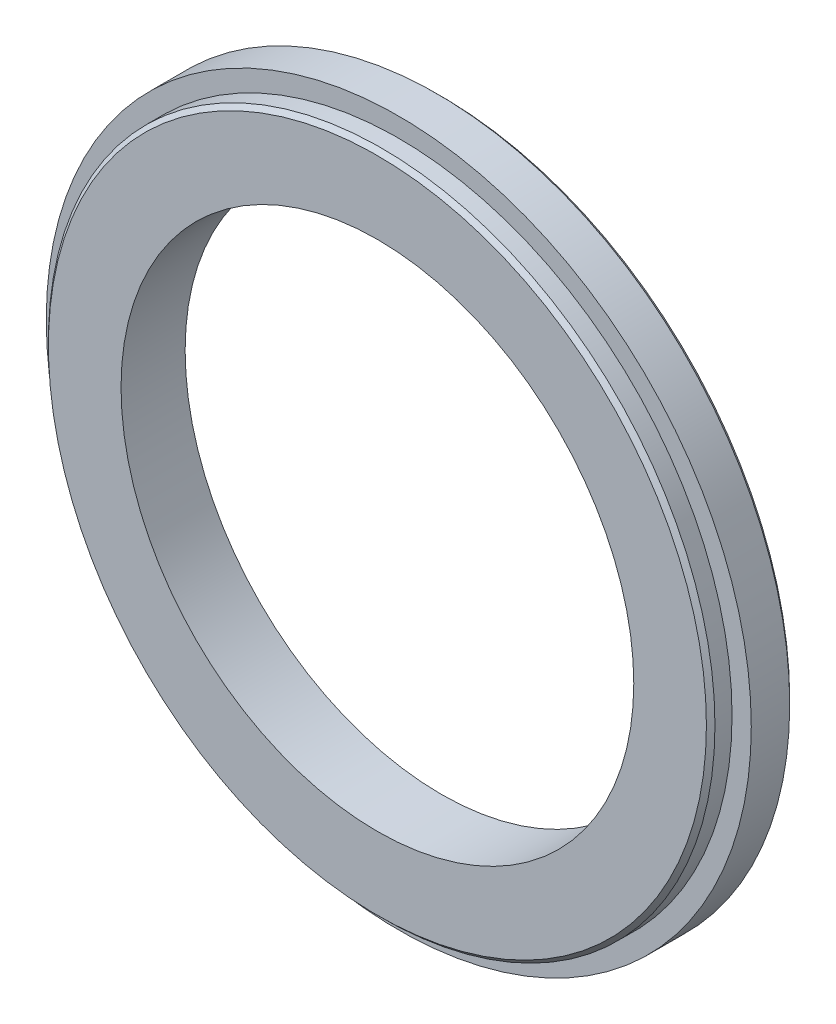
SolidWorks part; units mm, degrees
material "Plain carbon steel"
ref_plane "Front Plane" through (0, 0, 0) normal (0, 0, 1) x (1, 0, 0)
ref_plane "Top Plane" through (0, 0, 0) normal (0, 1, 0) x (1, 0, 0)
ref_plane "Right Plane" through (0, 0, 0) normal (1, 0, 0) x (0, 0, -1)
sketch "Sketch1" plane through (0, 0, 0) normal (0, 0, 1) x (1, 0, 0)
  circle A0 centre (0, 0) radius 82.5
  circle A1 centre (0, 0) radius 60
extrude "Boss-Extrude1" add sketch "Sketch1" along normal blind 10
sketch "Sketch2" plane through (0, 0, 10) normal (0, 0, 1) x (1, 0, 0)
  circle A0 centre (0, 0) radius 78
  circle A1 centre (0, 0) radius 60
extrude "Boss-Extrude2" add sketch "Sketch2" along normal blind 5
chamfer "Chamfer1" distance 1 distance2 1 2 edges at (82.5, 0, 0) (78, 0, 15)
sketch "Sketch3" plane through (0, 0, 0) normal (0, 0, -1) x (-1, 0, 0)
  circle A1 centre (70, 0) radius 3.95
  circle A2 centre (35, -60.6218) radius 3.95
  circle A3 centre (-35, -60.6218) radius 3.95
  circle A4 centre (-70, 0) radius 3.95
  circle A5 centre (-35, 60.6218) radius 3.95
  circle A6 centre (35, 60.6218) radius 3.95
  point P17 (0, 0)
  dimension "D1" = 6
hole_wizard "M8 Tapped Hole1" positions "3DSketch1" profile "Sketch4" tap size "M8" standard "Gb"
sketch3d "3DSketch1"
  point P0 (35, 60.6218, 0)
  point P3 (-35, 60.6218, 0)
  point P6 (-70, 0, 0)
  point P9 (-35, -60.6218, 0)
  point P12 (35, -60.6218, 0)
  point P15 (70, 0, 0)
sketch "Sketch4" plane through (35, 60.6218, 0) normal (1, 0, 0) x (0, 1, 0)
  line L0 (0, 0) -> (0, 14.0429)
  line L1 (0, 14.0429) -> (3.4, 12)
  line L2 (3.4, 12) -> (3.4, 0)
  line L5 (3.4, 0) -> (0, 0)
  line L10 (0, 14.0429) -> (-3.4, 12) construction
  line L11 (0, -6.35) -> (0, 107.95) construction
  dimension "螺纹孔钻头直径" = 6.8
  dimension "螺纹孔钻头深度" = 12
  dimension "导头角度" = 118
cosmetic thread "Hole Cosmetic Thread1" parameters "D1"=10, "D2"=8
cosmetic thread "Hole Cosmetic Thread2" parameters "D1"=10, "D2"=8
cosmetic thread "Hole Cosmetic Thread3" parameters "D1"=10, "D2"=8
cosmetic thread "Hole Cosmetic Thread4" parameters "D1"=10, "D2"=8
cosmetic thread "Hole Cosmetic Thread5" parameters "D1"=10, "D2"=8
cosmetic thread "Hole Cosmetic Thread6" parameters "D1"=10, "D2"=8
